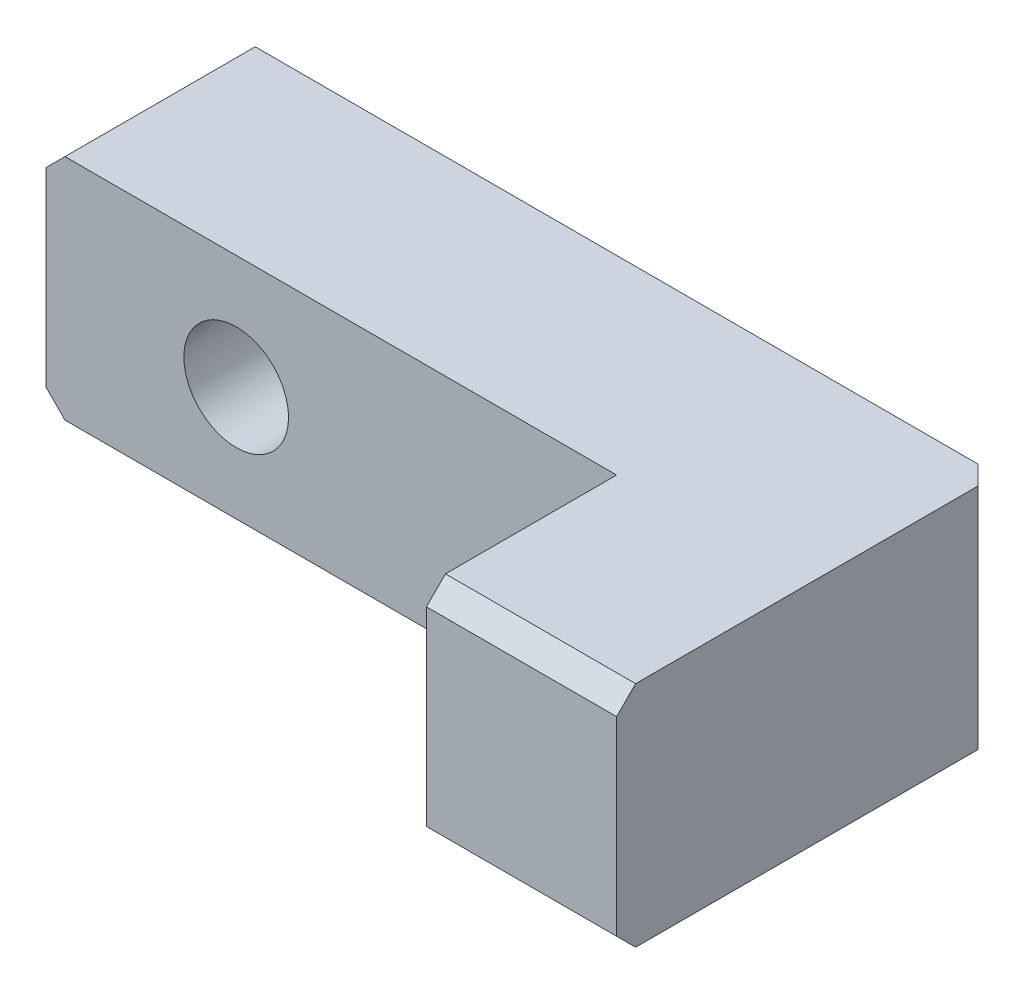
SolidWorks part; units mm, degrees
material "A6061"
ref_plane "前基準面" through (0, 0, 0) normal (0, 0, 1) x (1, 0, 0)
ref_plane "上基準面" through (0, 0, 0) normal (0, 1, 0) x (1, 0, 0)
ref_plane "右基準面" through (0, 0, 0) normal (1, 0, 0) x (0, 0, -1)
sketch "草图1" plane through (0, 0, 0) normal (0, 1, 0) x (1, 0, 0)
  line L1 (-20, -10) -> (20, -10)
  line L2 (-20, -10) -> (-20, 10)
  line L3 (-20, 10) -> (20, 10)
  line L4 (20, -10) -> (20, 10)
  line L5 (-20, -10) -> (20, 10) construction
  line L6 (-20, 10) -> (20, -10) construction
  point P0 (0, 0)
  dimension "D1" = 40
  dimension "D2" = 20
extrude "凸台-拉伸1" add sketch "草图1" along normal mid plane 12
sketch "草图2" plane through (0, 6, 0) normal (0, 1, 0) x (1, 0, 0)
  line L0 (20, 10) -> (-20, 10) construction
  line L1 (-20, -10) -> (10, -10)
  line L2 (-20, -10) -> (-20, 0)
  line L3 (-20, 0) -> (10, 0)
  line L4 (10, -10) -> (10, 0)
  line L5 (20, -10) -> (20, 10) construction
  dimension "D1" = 10
  dimension "D2" = 10
extrude "切除-拉伸1" cut sketch "草图2" against normal up to surface (12 mm away) up to face at (0, -6, 0)
hole_wizard "打孔尺寸(%根据)内六角圆柱头螺钉的类型1" positions "草图3" profile "草图4" counterbore size "M5" standard "GB" end condition through all
sketch "草图3" plane through (0, 0, -10) normal (0, 0, -1) x (-1, 0, 0)
  line L0 (-10, -6) -> (-10, 6) construction
  point P0 (10, 0)
  dimension "D1" = 20
sketch "草图4" plane through (-10, 0, -10) normal (1, 0, 0) x (0, 1, 0)
  line L0 (0, 0) -> (0, 20)
  line L1 (0, 20) -> (2.75, 20)
  line L3 (2.75, 20) -> (2.75, 5.7)
  line L4 (2.75, 5.7) -> (5, 5.7)
  line L5 (5, 5.7) -> (5, 0)
  line L7 (5, 0) -> (0, 0)
  line L11 (0, -6.35) -> (0, 107.95) construction
  dimension "通孔孔直径" = 5.5
  dimension "通孔孔深度" = 20
  dimension "柱形沉头孔直径" = 10
  dimension "柱形沉头孔深度" = 5.7
chamfer "倒角1" distance 1 angle 45 5 edges at (15, 6, 10) (15, -6, 10) (20, 0, -10) (-20, 6, -5) (-20, -6, -5)
